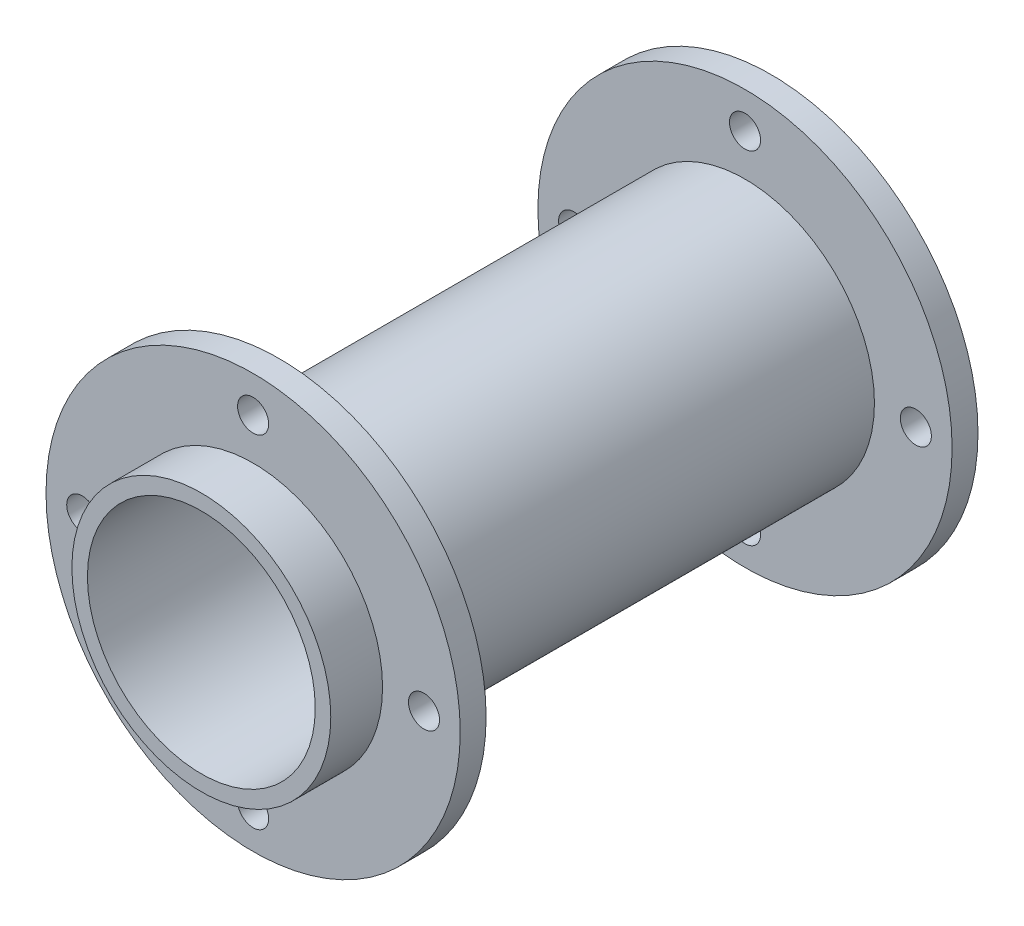
SolidWorks part; units mm, degrees
ref_plane "Front Plane" through (0, 0, 0) normal (0, 0, 1) x (1, 0, 0)
ref_plane "Top Plane" through (0, 0, 0) normal (0, 1, 0) x (1, 0, 0)
ref_plane "Right Plane" through (0, 0, 0) normal (1, 0, 0) x (0, 0, -1)
sketch "Sketch1" plane through (0, 0, 0) normal (0, 0, 1) x (1, 0, 0)
  circle A0 centre (0, 0) radius 25
  circle A1 centre (0, 0) radius 22
  dimension "D1" = 50
  dimension "D2" = 3
extrude "Boss-Extrude1" add sketch "Sketch1" along normal mid plane 120
sketch "Sketch2" plane through (0, 0, -60) normal (0, 0, -1) x (-1, 0, 0)
  circle A0 centre (0, 0) radius 25
  circle A1 centre (0, 0) radius 40
  circle A2 centre (0, 33) radius 3
  circle A3 centre (33, 0) radius 3
  circle A4 centre (0, -33) radius 3
  circle A5 centre (-33, 0) radius 3
  point P15 (0, 0)
  dimension "D1" = 33
  dimension "D2" = 6
  dimension "D3" = 80
  dimension "D4" = 4
extrude "Boss-Extrude2" add sketch "Sketch2" against normal blind 5 from offset 10 offset against normal yes
mirror "Mirror1" about plane through (0, 0, 0) normal (0, 0, 1) of "Boss-Extrude2"
